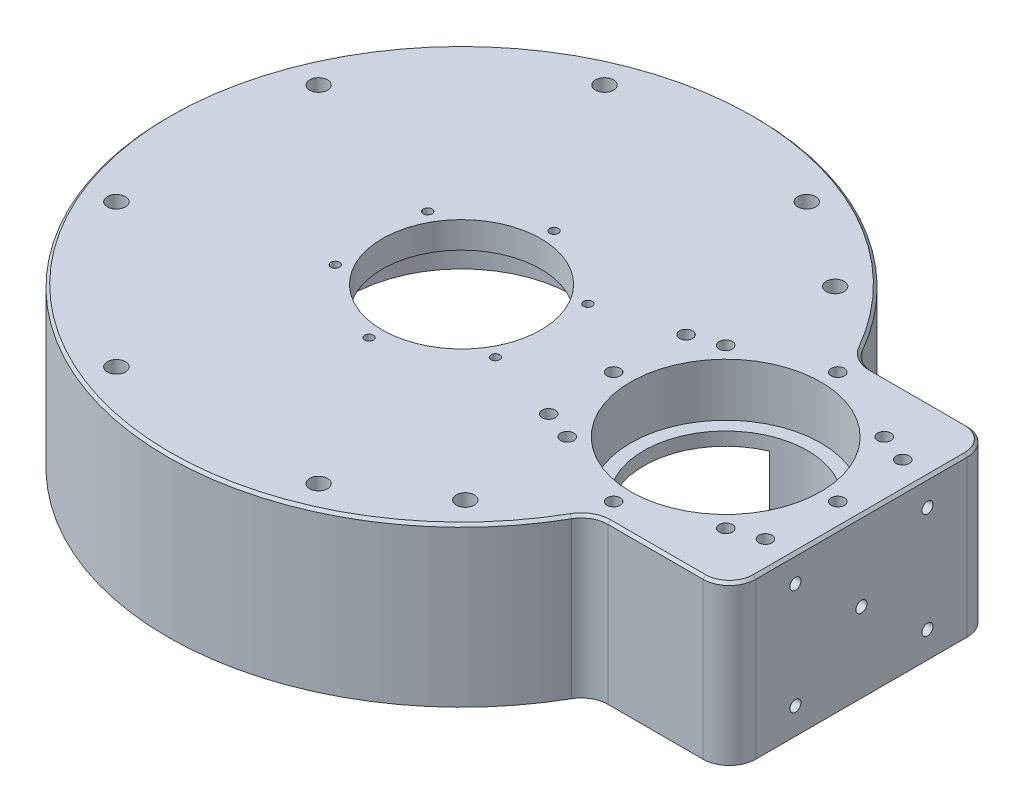
from build123d import *

# Parameters (mm, degrees)
SKETCH_2_W             = 52
SKETCH_2_H             = 100
EXTRUDE_1_DEPTH        = 60
SKETCH_3_R             = 36
CUT_EXTRUDE_1_DEPTH    = 20
SKETCH_4_R             = 31
CUT_EXTRUDE_2_DEPTH    = 24
SKETCH_9_R             = 95.5
SKETCH_9_R_2           = 92.5
EXTRUDE_2_DEPTH        = 3
HOLE_WIZARD_M8_3_D     = 6.8
HOLE_WIZARD_M8_3_DEPTH = 19.75
HOLE_WIZARD_M8_3_TIP   = 2.042926105
HOLE_WIZARD_M6_1_D     = 5
HOLE_WIZARD_M6_1_DEPTH = 15
HOLE_WIZARD_M6_1_TIP   = 1.502151548
CUT_EXTRUDE_4_DEPTH    = 3
EXTRUDE_START          = -10
SKETCH_18_R            = 39.5
SKETCH_18_R_2          = 30
EXTRUDE_3_DEPTH        = 10
HOLE_WIZARD_M4_1_D     = 3.3
HOLE_WIZARD_M4_1_DEPTH = 8
HOLE_WIZARD_M4_1_TIP   = 0.991420021
HOLE_WIZARD_M8_5_D     = 6.8
HOLE_WIZARD_M8_5_DEPTH = 19.75
HOLE_WIZARD_M8_5_TIP   = 2.042926105
FILLET_1_R             = 10
CHAMFER_1_SIZE         = 1
HOLE_WIZARD_M5_1_D     = 4.2
HOLE_WIZARD_M5_1_DEPTH = 12.4
HOLE_WIZARD_M5_1_TIP   = 1.2618073


with BuildPart() as part:
    # 草图1 → 旋转1 (revolve)
    with BuildSketch(Plane.XY, mode=Mode.PRIVATE) as revolve_1_sk:
        Polygon((92.5, 0), (111.25, 0), (111.25, 60), (39.5, 60), (39.5, 45), (42.5, 45), (42.5, 35), (92.5, 35), align=None)
    revolve(revolve_1_sk.sketch.rotate(Axis((0, 0, 0), (0, 1, 0)), 90), axis=Axis((0, 0, 0), (0, 1, 0)))

    # 草图2 → 凸台-拉伸1 (add, through all)
    with BuildSketch(Plane.XZ):
        with Locations((125.380896052, 0)):
            Rectangle(SKETCH_2_W, SKETCH_2_H)
    extrude(amount=-EXTRUDE_1_DEPTH)

    # 草图3 → 切除-拉伸1 (cut)
    with BuildSketch(Plane(origin=(0, 60, 0), x_dir=(1, 0, 0), z_dir=(0, 1, 0))):
        with Locations(Location((100, 0, 0), (0, 0, 270))):
            Circle(SKETCH_3_R)
    extrude(amount=-CUT_EXTRUDE_1_DEPTH, mode=Mode.SUBTRACT)

    # 草图4 → 切除-拉伸2 (cut)
    with BuildSketch(Plane(origin=(0, 40, 0), x_dir=(1, 0, 0), z_dir=(0, 1, 0))):
        with Locations(Location((100, 0, 0), (0, 0, 270))):
            Circle(SKETCH_4_R)
    extrude(amount=-CUT_EXTRUDE_2_DEPTH, mode=Mode.SUBTRACT)

    # 草图9 → 凸台-拉伸2 (add)
    with BuildSketch(Plane(origin=(0, 16, 0), x_dir=(1, 0, 0), z_dir=(0, 1, 0))):
        Circle(SKETCH_9_R)
        with Locations(Location((0, 0, 0), (0, 0, 90))):
            Circle(SKETCH_9_R_2, mode=Mode.SUBTRACT)
    extrude(amount=EXTRUDE_2_DEPTH)

    # M8 螺纹孔3
    with Locations(Plane(origin=(0, 0, 0), x_dir=(-1, 0, 0), z_dir=(0, -1, 0))):
        with Locations((39.799076966, 96.083471381), (96.083471381, 39.799076966), (96.083471381, -39.799076966), (39.799076966, -96.083471381), (-39.799076966, -96.083471381), (-96.083471381, -39.799076966), (-96.083471381, 39.799076966), (-39.799076966, 96.083471381)):
            Hole(HOLE_WIZARD_M8_3_D / 2, depth=HOLE_WIZARD_M8_3_DEPTH)
            with Locations((0, 0, -(HOLE_WIZARD_M8_3_DEPTH + HOLE_WIZARD_M8_3_TIP / 2))):  # 118° drill point
                Cone(0, HOLE_WIZARD_M8_3_D / 2, HOLE_WIZARD_M8_3_TIP, mode=Mode.SUBTRACT)

    # M6 螺纹孔1
    with Locations(Plane(origin=(0, 60, 0), x_dir=(1, 0, 0), z_dir=(0, 1, 0))):
        with Locations((70, 30), (130, 30), (130, -30), (70, -30), (100, 0), (100, 42.426406871), (100, -42.426406871), (57.573593129, 0), (142.426406871, 0), (59, -26), (59, 26), (141, 26), (141, -26)):
            Hole(HOLE_WIZARD_M6_1_D / 2, depth=HOLE_WIZARD_M6_1_DEPTH)
            with Locations((0, 0, -(HOLE_WIZARD_M6_1_DEPTH + HOLE_WIZARD_M6_1_TIP / 2))):  # 118° drill point
                Cone(0, HOLE_WIZARD_M6_1_D / 2, HOLE_WIZARD_M6_1_TIP, mode=Mode.SUBTRACT)

    # 草图17 → 切除-拉伸4 (cut)
    with BuildSketch(Plane(origin=(0, 19, 0), x_dir=(1, 0, 0), z_dir=(0, 1, 0))):
        with BuildLine():
            ThreePointArc((87.97625, -28.573229358), (89.373787568, -29.1218751), (90.79625, -29.602212518))
            ThreePointArc((90.79625, -29.602212518), (95.5, 0), (90.79625, 29.602212518))
            ThreePointArc((90.79625, 29.602212518), (89.373787568, 29.1218751), (87.97625, 28.573229358))
            ThreePointArc((87.97625, 28.573229358), (92.5, 0), (87.97625, -28.573229358))
        make_face()
    extrude(amount=-CUT_EXTRUDE_4_DEPTH, mode=Mode.SUBTRACT)

    # 草图18 → 凸台-拉伸3 (add)
    with BuildSketch(Plane(origin=(0, 60, 0), x_dir=(1, 0, 0), z_dir=(0, 1, 0)).offset(EXTRUDE_START)):
        with Locations(Location((0, 0, 0), (0, 0, 90))):
            Circle(SKETCH_18_R)
        with Locations(Location((0, 0, 0), (0, 0, 270))):
            Circle(SKETCH_18_R_2, mode=Mode.SUBTRACT)
    extrude(amount=EXTRUDE_3_DEPTH)

    # M4 螺纹孔1
    with Locations(Plane(origin=(0, 60, 0), x_dir=(1, 0, 0), z_dir=(0, 1, 0))):
        with Locations((0, 35), (30.310889132, 17.5), (30.310889132, -17.5), (0, -35), (-30.310889132, -17.5), (-30.310889132, 17.5)):
            Hole(HOLE_WIZARD_M4_1_D / 2, depth=HOLE_WIZARD_M4_1_DEPTH)
            with Locations((0, 0, -(HOLE_WIZARD_M4_1_DEPTH + HOLE_WIZARD_M4_1_TIP / 2))):  # 118° drill point
                Cone(0, HOLE_WIZARD_M4_1_D / 2, HOLE_WIZARD_M4_1_TIP, mode=Mode.SUBTRACT)

    # M8 螺纹孔5
    with Locations(Plane(origin=(0, 60, 0), x_dir=(1, 0, 0), z_dir=(0, 1, 0))):
        with Locations((38.268343237, 92.387953251), (38.268343237, -92.387953251), (-38.268343237, -92.387953251), (-92.387953251, -38.268343237), (-92.387953251, 38.268343237), (-38.268343237, 92.387953251), (71.414284285, 70), (71.414284285, -70)):
            Hole(HOLE_WIZARD_M8_5_D / 2, depth=HOLE_WIZARD_M8_5_DEPTH)
            with Locations((0, 0, -(HOLE_WIZARD_M8_5_DEPTH + HOLE_WIZARD_M8_5_TIP / 2))):  # 118° drill point
                Cone(0, HOLE_WIZARD_M8_5_D / 2, HOLE_WIZARD_M8_5_TIP, mode=Mode.SUBTRACT)

    # 圆角1
    fillet_1_edges = [part.edges().sort_by_distance(p)[0] for p in [
        (99.380896052, 30, -50),
        (99.380896052, 30, 50),
        (151.380896052, 30, 50),
        (151.380896052, 30, -50),
    ]]
    fillet(fillet_1_edges, radius=FILLET_1_R)

    # 倒角1
    chamfer_1_edges = [part.edges().sort_by_distance(p)[0] for p in [
        (123.372424308, 60, 50),
        (-111.25, 60, 0),
        (123.372424308, 60, -50),
        (151.380896052, 60, 0),
        (148.451963863, 60, 47.071067812),
        (148.451963863, 60, -47.071067812),
        (100.338245454, 60, 51.354638929),
        (100.338245454, 60, -51.354638929),
    ]]
    chamfer(chamfer_1_edges, length=CHAMFER_1_SIZE)

    # M5 螺纹孔1
    with Locations(Plane(origin=(151.380896052, 0, 0), x_dir=(0, 0, -1), z_dir=(1, 0, 0))):
        with Locations((-25, 50), (0, 30), (25, 50), (-25, 10), (25, 10)):
            Hole(HOLE_WIZARD_M5_1_D / 2, depth=HOLE_WIZARD_M5_1_DEPTH)
            with Locations((0, 0, -(HOLE_WIZARD_M5_1_DEPTH + HOLE_WIZARD_M5_1_TIP / 2))):  # 118° drill point
                Cone(0, HOLE_WIZARD_M5_1_D / 2, HOLE_WIZARD_M5_1_TIP, mode=Mode.SUBTRACT)


solid = part.part
